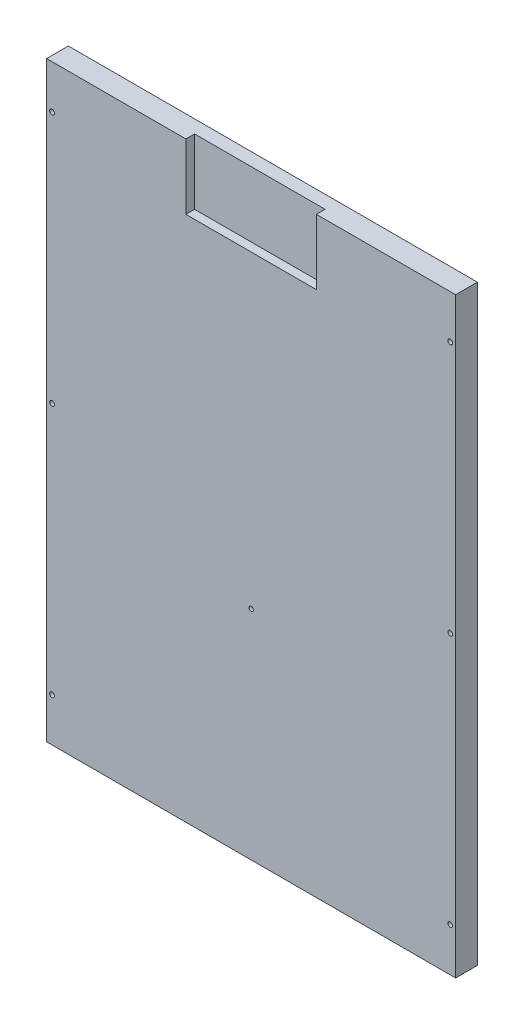
from build123d import *

# Parameters (mm, degrees)
SKETCH_1_W            = 940
SKETCH_1_H            = 1360
EXTRUDE_1_DEPTH       = 50
SKETCH_2_R            = 5
SKETCH_2_R_2          = 5.5
SKETCH_2_W            = 300
SKETCH_2_H            = 300
CUT_EXTRUDE_986_DEPTH = 20


with BuildPart() as part:
    # 草图1 → 凸台-拉伸1 (new body)
    with BuildSketch(Plane.XY):
        Rectangle(SKETCH_1_W, SKETCH_1_H)
    extrude(amount=EXTRUDE_1_DEPTH)

    # 草图2 → Cut-Extrude 986 (cut)
    with BuildSketch(Plane.XY.offset(50)):
        with Locations((0, -180)):
            Circle(SKETCH_2_R)
        with Locations((457.5, -580)):
            Circle(SKETCH_2_R_2)
        with Locations((457.5, 0)):
            Circle(SKETCH_2_R_2)
        with Locations((457.5, 580)):
            Circle(SKETCH_2_R_2)
        with Locations(Location((-457.5, 580, 0), (0, 0, 180))):
            Circle(SKETCH_2_R_2)
        with Locations(Location((-457.5, 0, 0), (0, 0, 180))):
            Circle(SKETCH_2_R_2)
        with Locations(Location((-457.5, -580, 0), (0, 0, 180))):
            Circle(SKETCH_2_R_2)
        with Locations((0, 680)):
            Rectangle(SKETCH_2_W, SKETCH_2_H)
    extrude(amount=-CUT_EXTRUDE_986_DEPTH, mode=Mode.SUBTRACT)


solid = part.part
